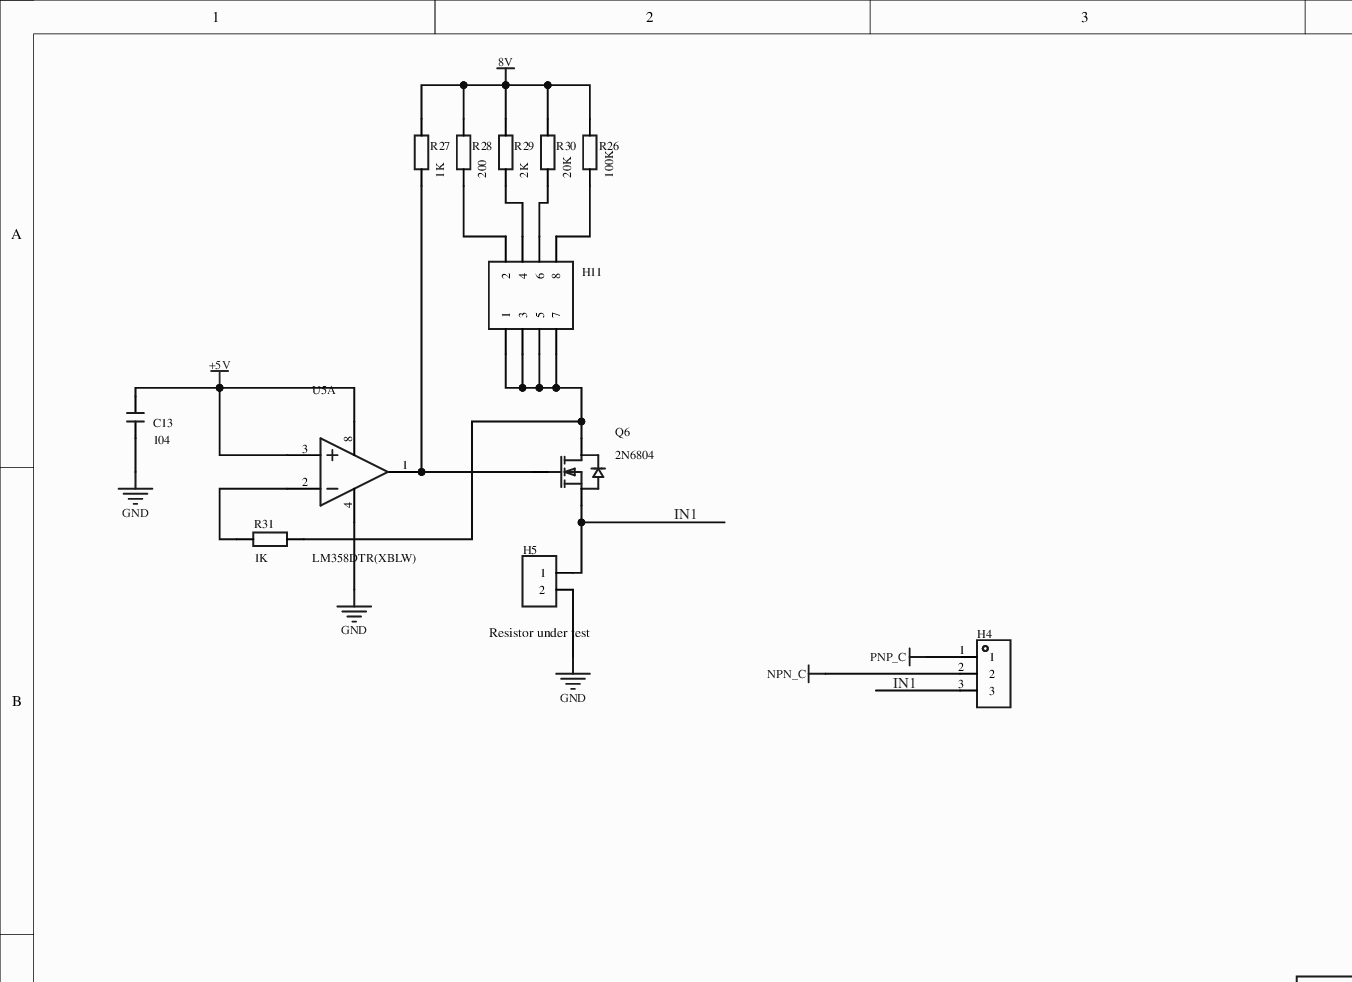
[diagram p0: MISC52056-3.schdoc, top left]
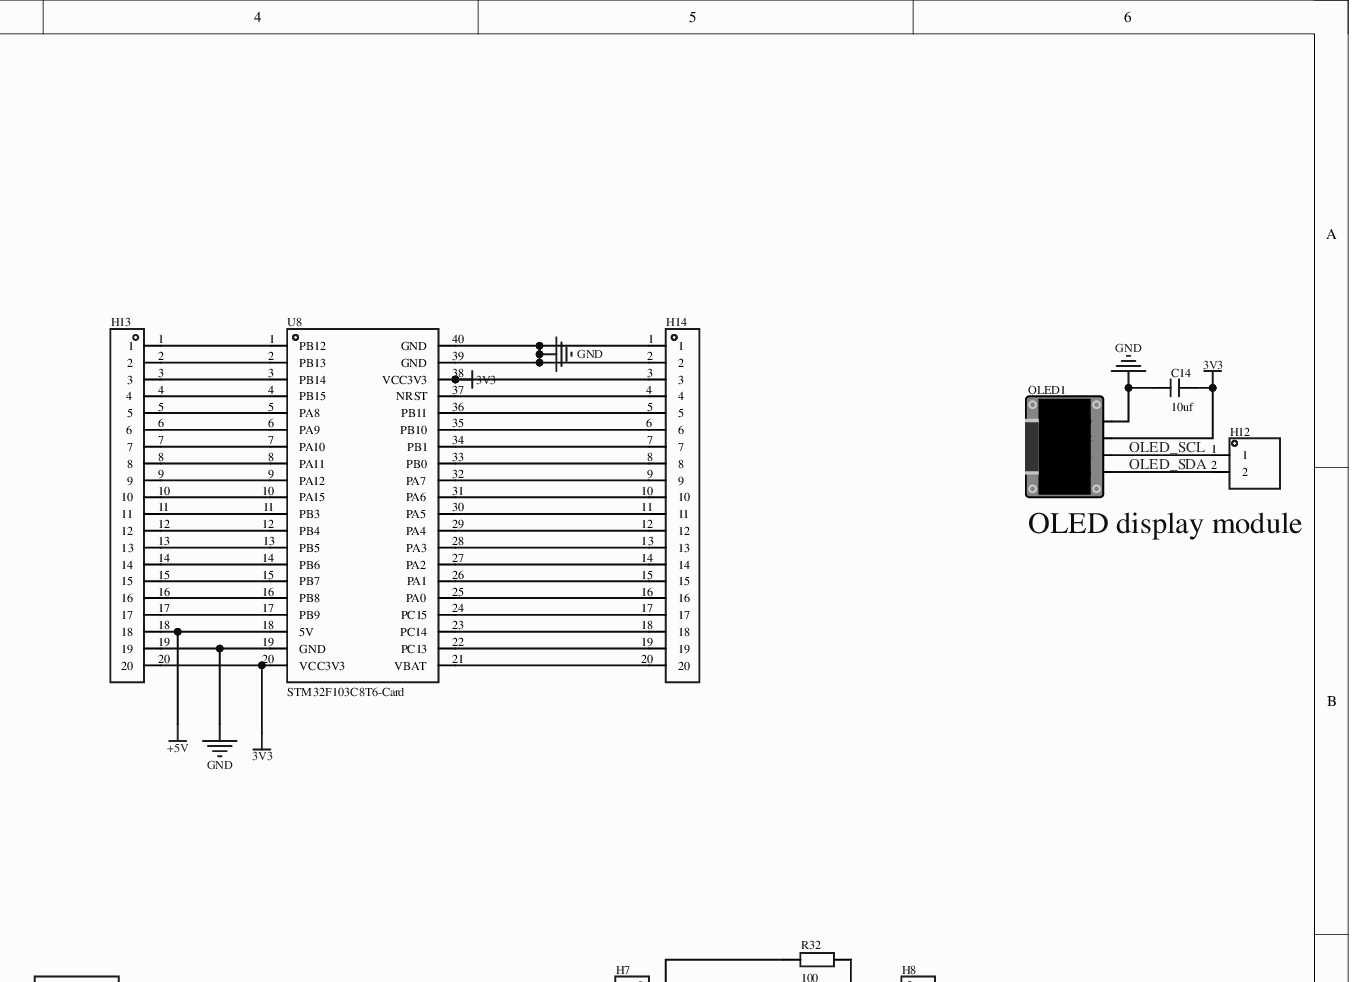
[diagram p1: MISC52056-3.schdoc, top right]
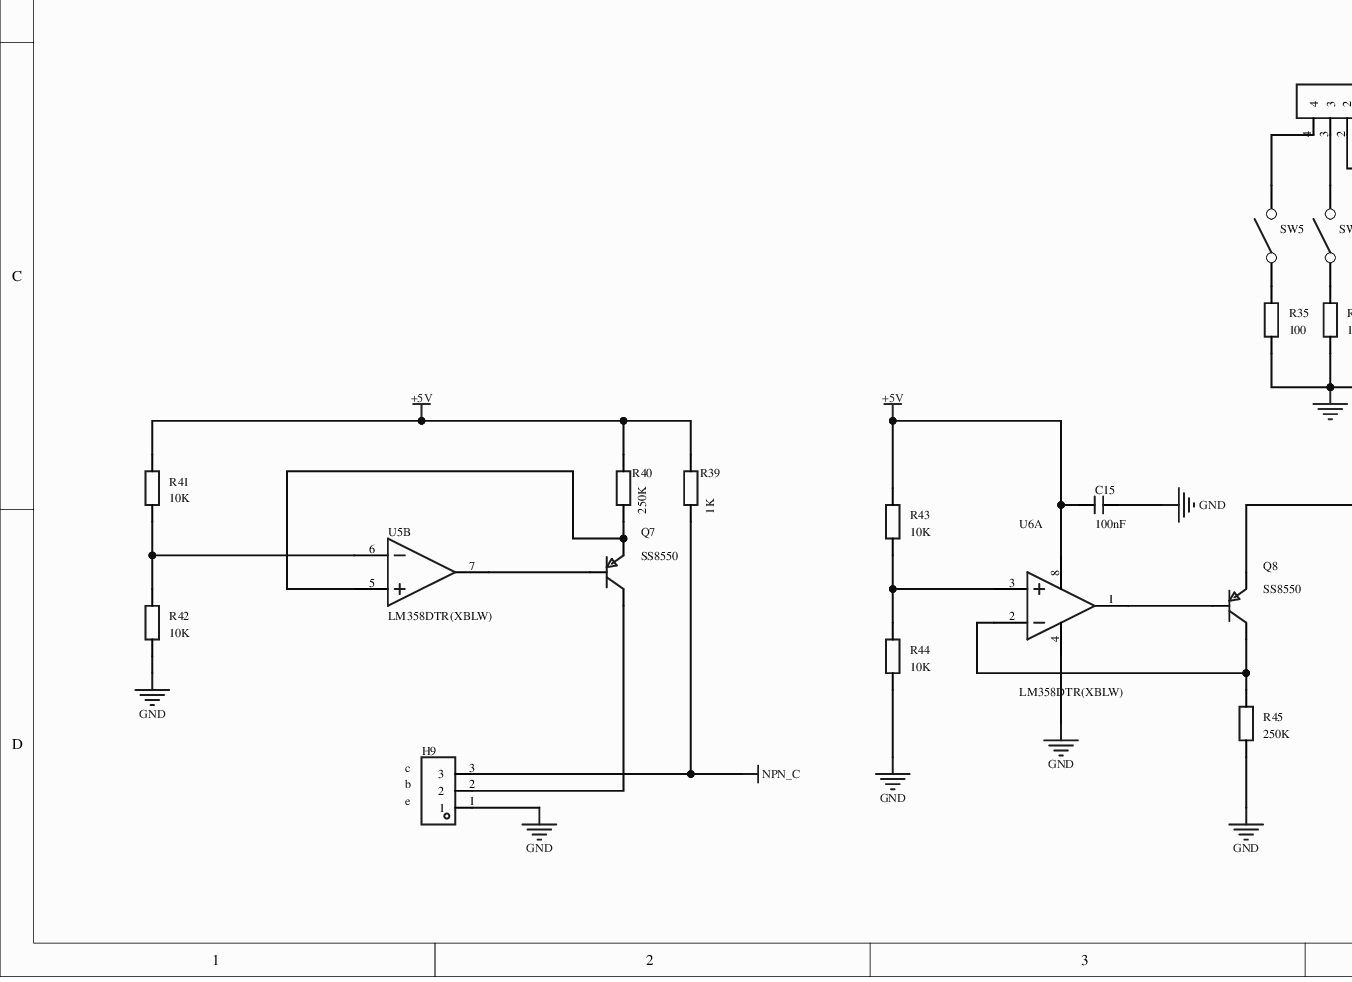
[diagram p2: MISC52056-3.schdoc, bottom left]
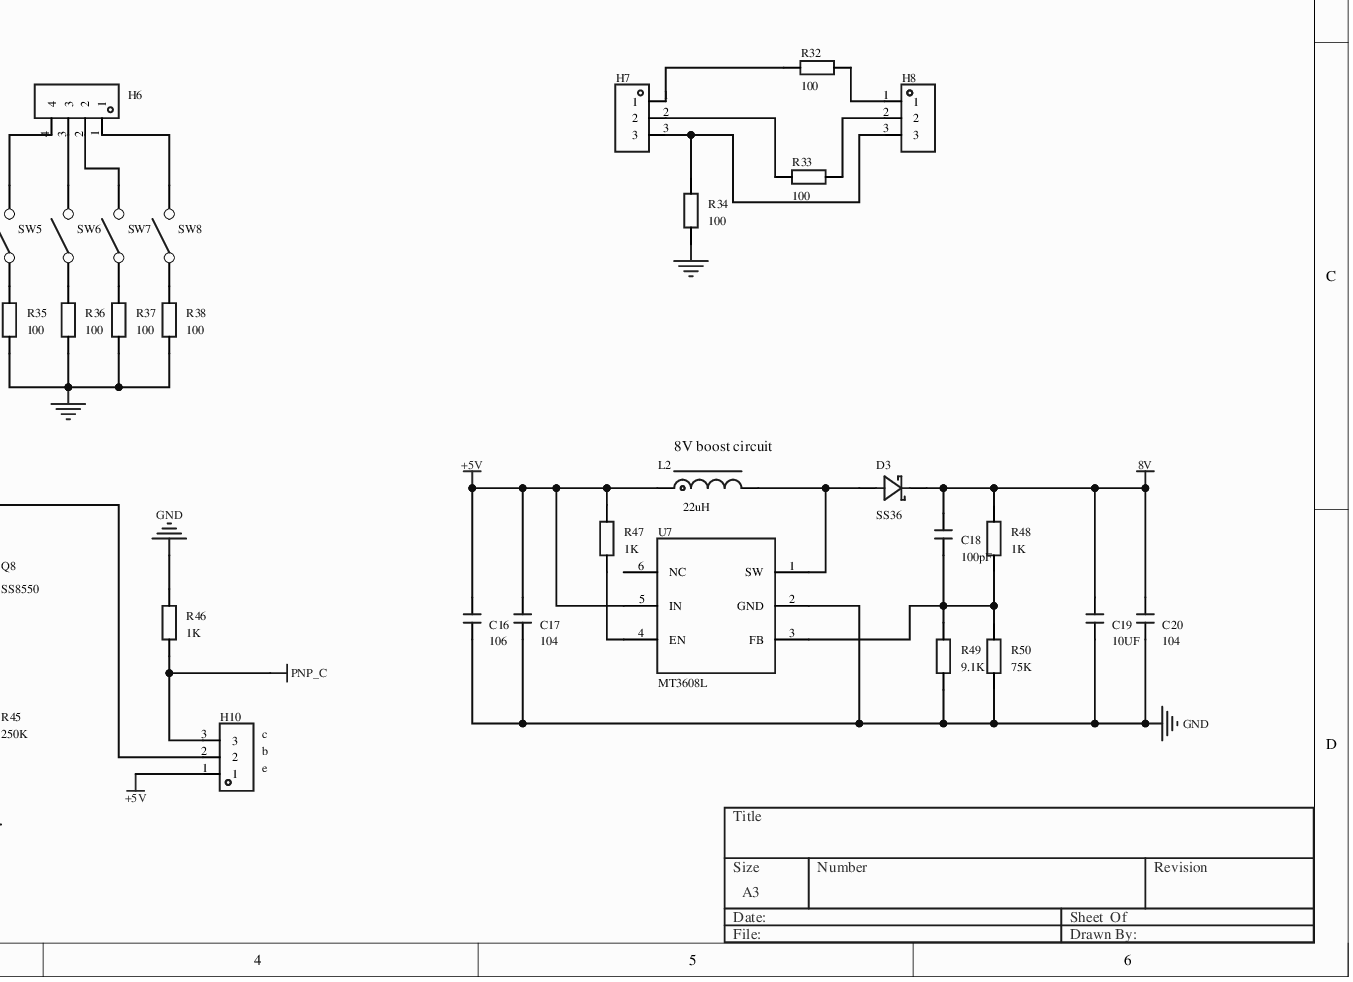
[diagram p3: MISC52056-3.schdoc, bottom right]
# Altium project MISC52056-2.PrjPcb
1 sheet, 58 parts. Net scope: global (net labels, ports and power ports of the same name join across sheets).
Board file: MISC52056.pcbdoc

## Sheet MISC52056-3.schdoc
size 393 x 282 mm; @Page No: 1; @Page Count: 1; @Schematic Name: MISC52056; @Project Name: MISC52056; @Board Name: MISC52056; @Update Date: 2025-02-22; @Create Time: 23:15:00; @Update Time: 00:31:48; @Create Date: 2025-02-22

### Parts
C13  104  [C0603]
C14  10uf  [C0603]
C15  100nF  [C0603]
C16  106  [C0603]
C17  104  [C0603]
C18  100pF  [C0603]
C19  10UF  [C0603]
C20  104  [C0603]
D3  SS36  [SMA_L4.3-W2.6-LS5.0-FD]
H4  (no value)  [HDR-TH_3P-P2.54-V-F]
H5  (no value)  [HDR-TH_2P-P2.54-V-F]
H6  (no value)  [HDR-TH_4P-P2.54-V-M]
H7  (no value)  [HDR-TH_3P-P2.54-V-F]
H8  (no value)  [HDR-TH_3P-P2.54-V-F]
H9  (no value)  [HDR-TH_3P-P2.54-V-F]
H10  (no value)  [HDR-TH_3P-P2.54-V-F]
H11  (no value)  [HDR-TH_8P-P2.54-V-M-R2-C4-S2.54]
H12  (no value)  [HDR-TH_2P-P2.54-V-M-1]
H13  (no value)  [HDR-TH_20P-P2.54-V-M-1]
H14  (no value)  [HDR-TH_20P-P2.54-V-M-1]
L2  22uH  [IND-SMD_L7.1-W6.6]
OLED1  (no value)  [0.96OLED_4P]
Q6  2N6804  [TO-220-3_L10.0-W4.5-P2.54-L]
Q7  SS8550  [SOT-23-3_L2.9-W1.3-P1.90-LS2.4-BR]
Q8  SS8550  [SOT-23-3_L2.9-W1.3-P1.90-LS2.4-BR]
R26  100K  [R0603]
R27  1K  [R0603]
R28  200  [R0603]
R29  2K  [R0603]
R30  20K  [R0603]
R31  1K  [R0603]
R32  100  [R0603]
R33  100  [R0603]
R34  100  [R0603]
R35  100  [R0603]
R36  100  [R0603]
R37  100  [R0603]
R38  100  [R0603]
R39  1K  [R0603]
R40  250K  [R0603]
R41  10K  [R0603]
R42  10K  [R0603]
R43  10K  [R0603]
R44  10K  [R0603]
R45  250K  [R0603]
R46  1K  [R0603]
R47  1K  [R0603]
R48  1K  [R0603]
R49  9.1K  [R0603]
R50  75K  [R0603]
SW5  TS-1088-AR02016  [SW-SMD_L3.9-W3.0-P4.45]  (value not drawn)
SW6  TS-1088-AR02016  [SW-SMD_L3.9-W3.0-P4.45]  (value not drawn)
SW7  TS-1088-AR02016  [SW-SMD_L3.9-W3.0-P4.45]  (value not drawn)
SW8  TS-1088-AR02016  [SW-SMD_L3.9-W3.0-P4.45]  (value not drawn)
U5  LM358DTR(XBLW)  [SOIC-8_L4.9-W4.0-P1.27-LS6.0-BL]  (parts A,B of 2)
U6  LM358DTR(XBLW)  [SOIC-8_L4.9-W4.0-P1.27-LS6.0-BL]  (part A of 2)
U7  MT3608L  [SOT-23-6_L2.9-W1.6-P0.95-LS2.8-BL_3]
U8  STM32F103C8T6-Card  [CONN-TH_L53.3-W22.9_STM32F103C8T6-CARD]

### Nets
3V3: C14.1 H13.20 H14.3 OLED1.2(VCC) U8.20(VCC3V3) U8.38(VCC3V3)
GND: C13.1 C14.2 C15.1 C16.2 C17.2 C19.2 C20.2 H5.2 H9.1 H13.19 H14.1 H14.2 OLED1.1(GND) R34.2 R35.2 R36.2 R37.2 R38.2 R42.1 R44.1 R45.1 R46.2 R49.1 R50.1 U5.4(V-) U6.4(V-) U7.2(GND) U8.19(GND) U8.39(GND) U8.40(GND)  [also labelled 5V, E]
8V: C18.1 C19.1 C20.1 D3.2(K) R26.2 R27.2 R28.2 R29.2 R30.2 R48.1
+5V: C13.2 C15.2 C16.1 C17.1 H10.1 H13.18 L2.1 R39.2 R40.2 R41.2 R43.2 R47.2 U5.3(IN+) U5.8(V+) U6.8(V+) U7.5(IN) U8.18(5V)
NPN_C: H4.1 H4.2 H9.3 H10.3 R39.1 R46.1  [also labelled C, PNP_C]
IN1: H4.3 H5.1 Q6.3(S)
OLED_SCL: H12.1 OLED1.3(SCL)
OLED_SDA: H12.2 OLED1.4(SDA)
NetC18_2: C18.2 R48.2 R49.2 R50.2 U7.3(FB)
NetD3_1: D3.1(A) L2.2 U7.1(SW)
NetH6_1: H6.1 SW8.2(NO)
NetH6_2: H6.2 SW7.2(NO)
NetH6_3: H6.3 SW6.2(NO)
NetH6_4: H6.4 SW5.2(NO)
NetH7_1: H7.1 R32.2
NetH7_2: H7.2 R33.2
NetH7_3: H7.3 H8.3 R34.1
NetH8_1: H8.1 R32.1
NetH8_2: H8.2 R33.1
NetH9_2: H9.2 Q7.3(C)
NetH10_2: H10.2 Q8.2(E)
NetH11_1: H11.1 H11.3 H11.5 H11.7 Q6.2(D) R31.1
NetH11_2: H11.2 R28.1
NetH11_4: H11.4 R29.1
NetH11_6: H11.6 R30.1
NetH11_8: H11.8 R26.1
NetH13_1: H13.1 U8.1(PB12)
NetH13_2: H13.2 U8.2(PB13)
NetH13_3: H13.3 U8.3(PB14)
NetH13_4: H13.4 U8.4(PB15)
NetH13_5: H13.5 U8.5(PA8)
NetH13_6: H13.6 U8.6(PA9)
NetH13_7: H13.7 U8.7(PA10)
NetH13_8: H13.8 U8.8(PA11)
NetH13_9: H13.9 U8.9(PA12)
NetH13_10: H13.10 U8.10(PA15)
NetH13_11: H13.11 U8.11(PB3)
NetH13_12: H13.12 U8.12(PB4)
NetH13_13: H13.13 U8.13(PB5)
NetH13_14: H13.14 U8.14(PB6)
NetH13_15: H13.15 U8.15(PB7)
NetH13_16: H13.16 U8.16(PB8)
NetH13_17: H13.17 U8.17(PB9)
NetH14_4: H14.4 U8.37(NRST)
NetH14_5: H14.5 U8.36(PB11)
NetH14_6: H14.6 U8.35(PB10)
NetH14_7: H14.7 U8.34(PB1)
NetH14_8: H14.8 U8.33(PB0)
NetH14_9: H14.9 U8.32(PA7)
NetH14_10: H14.10 U8.31(PA6)
NetH14_11: H14.11 U8.30(PA5)
NetH14_12: H14.12 U8.29(PA4)
NetH14_13: H14.13 U8.28(PA3)
NetH14_14: H14.14 U8.27(PA2)
NetH14_15: H14.15 U8.26(PA1)
NetH14_16: H14.16 U8.25(PA0)
NetH14_17: H14.17 U8.24(PC15)
NetH14_18: H14.18 U8.23(PC14)
NetH14_19: H14.19 U8.22(PC13)
NetH14_20: H14.20 U8.21(VBAT)
NetQ6_1: Q6.1(G) R27.1 U5.1(OUT)
NetQ7_1: Q7.1(B) U5.7(OUT_B)
NetQ7_2: Q7.2(E) R40.1 U5.5(IN_B+)
NetQ8_1: Q8.1(B) U6.1(OUT)
NetQ8_3: Q8.3(C) R45.2 U6.2(IN-)
NetR31_2: R31.2 U5.2(IN-)
NetR35_1: R35.1 SW5.1(COMMON)
NetR36_1: R36.1 SW6.1(COMMON)
NetR37_1: R37.1 SW7.1(COMMON)
NetR38_1: R38.1 SW8.1(COMMON)
NetR41_1: R41.1 R42.2 U5.6(IN_B-)
NetR43_1: R43.1 R44.2 U6.3(IN+)
NetR47_1: R47.1 U7.4(EN)

Not connected (* = marked no-connect by the designer): U7 6(NC)

### Notes on the sheet
- OLED display module
- (near H5) Resistor under test
- (near L2) 8V boost circuit
- (near H10) c
- (near H10) b
- (near H9) c
- (near H9) b
- (near H9) e
- (near H10) e
- Title
- File:
- Date:
- Size
- A3
- Number
- Drawn By:
- Sheet
- Of
- Revision

### Library data of the parts
C13-C20 = CAP_0603: ConvertToPcb: yes; SymbolName: CapAcitance; ModelId: ac125912035d415993ca9572d50418b1; ModelName: C0603_L1.6-W0.8-H0.8; ModelTransform: 62.992,31.496,0,0,0,0,0,0,0; Device: CAP_0603; AddInBom: yes; Supplier Footprint: 0603; FootprintName: C0603
  C13 C17 C20: Value: 104
  C14: Value: 10uf
  C15: Value: 100nF
  C16: Value: 106
  C18: Value: 100pF
  C19: Value: 10UF
D3 = SS36_C7420367: Diode configuration: discrete; forward voltage drop (Vf): 700mV@3.0A; DC reverse voltage (Vr): 60V; rectifier current: 3A;; Manufacturer: 宏迦橙; AddInBom: yes; ModelId: 7e24bebe6cd74171ae8c9de6fc5b78aa; ModelTransform: 198.4248,103.5431,0,180,0,0,0,0,0; Reverse Leakage Current (Ir): 10mA@60V; Symbol: SS36_C7420367; Device: SS36_C7420367; LCSC Part Name: 电压:60V 电流:3A; SupplierPart: C7420367; ManufacturerPart: SS36; Supplier Footprint: SMA(DO-214AC); JLCPCB Part Class: Extended library; Datasheet: example.com/20230828/75438452AEE6C276EDA92B2AF599BE05.pdf; Supplier: LCSC; ConvertToPcb: yes; FootprintName: SMA_L4.3-W2.6-LS5.0-FD; ModelName: SMA_L4.3-W2.6-LS5.0-FD; Diode Configuration: Discrete; Forward Voltage (Vf@If): 700mV@3.0A; Reverse Voltage (Vr): 60V; Rectified Current: 3A
H4 H7-H10 = HDR-F_2.54_1x3P: Symbol: PM254V-11-03-H85; ConvertToPcb: yes; ModelId: f3b3cc5aae9641bf9e56fc160cef875b; ModelName: HDR2.54-F-LI-1X3P; ModelTransform: 299.9994,100,0,0,0,0,0,0,-118.11; Device: HDR-F_2.54_1x3P; AddInBom: yes; SupplierPart: C541850; Supplier Footprint: 插件; FootprintName: HDR-TH_3P-P2.54-V-F
H5 = HDR-F_2.54_1x2P: Symbol: Header-Female-2.54_1x2; ConvertToPcb: yes; ModelId: a9450ef445564560a104363b9aacde4e; ModelName: HDR-TH_2P-P2.54-F-LI-1X2P; ModelTransform: 215.7476,98.425,0,0,0,0,0,0,-129.921; Device: HDR-F_2.54_1x2P; AddInBom: yes; SupplierPart: C49661; Supplier Footprint: 插件; FootprintName: HDR-TH_2P-P2.54-V-F
H6 = HDR-M_2.54_1x4P: Symbol: PZ254V-11-04P; ConvertToPcb: yes; ModelId: 112f4d05e8d64e99ab9a333894bea4f9; ModelName: HDR-TH_4P-P2.54-M-LI-1X4P; ModelTransform: 399.999,104.7242,0,0,0,0,0,0,-118.11; Device: HDR-M_2.54_1x4P; AddInBom: yes; SupplierPart: C492403; Supplier Footprint: 插件; FootprintName: HDR-TH_4P-P2.54-V-M
H11 = HDR-M_2.54_2x4: Symbol: HDR-M-2.54_2x4; ConvertToPcb: yes; ModelId: 9655140a9899454ea9d6a6732d55fb0e; ModelName: HDR-TH_8P-P2.54-M-LI-2X4P; ModelTransform: 399.999,200,0,0,0,0,0,0,-118.11; Device: HDR-M_2.54_2x4; AddInBom: yes; SupplierPart: C124386; Supplier Footprint: 插件,P=2.54mm; FootprintName: HDR-TH_8P-P2.54-V-M-R2-C4-S2.54
H12 = HDR-M_2.54_1x2P: Symbol: 210S-1*2P L=11.6MMGold-plated black; ConvertToPcb: yes; ModelId: 79b2e9f2d70a4d68a1b7098f27c6d4c5; ModelName: HDR-M-2.54_1x2; ModelTransform: 200,100,0,0,0,0,0,0,-118.11; Device: HDR-M_2.54_1x2P; AddInBom: yes; SupplierPart: C124375; Supplier Footprint: 插件; FootprintName: HDR-TH_2P-P2.54-V-M-1
H13 H14 = HDR-M_2.54_1x20P: Pitch: 2.54mm; total pin count: 20; rows: 1; pin structure: -; row spacing: -; mounting type: through-hole; round/square pin: -; rated current: -; rated voltage: -; mating pin length: -; plastic height: -; contact material: brass; contact plating: -; colour: black;; Symbol: HDR_2.54-1x20P; ConvertToPcb: yes; ModelId: f68709be121d406db68b06f32a595389; ModelName: HDR-M-2.54_1x20; ModelTransform: 1999.996,100,0,0,0,0,0,0,-118.11; Device: HDR-M_2.54_1x20P; AddInBom: yes; SupplierPart: C50981; Supplier Footprint: 插件; FootprintName: HDR-TH_20P-P2.54-V-M-1
L2 = YSPI0630A-220M: Inductance: 22uH; tolerance: ±20%; rated current: 3A;; Manufacturer: YJYCOIN(益嘉源); AddInBom: yes; DC Resistance (DCR): 130mΩ; ModelId: f4ba7fb6b518404398a5bef98cb0da31; ModelName: IND-SMD_L6.6-W7.1-H3.0; ModelTransform: 275.59,263.779,0,0,0,0,0,0.0005,0; Symbol: YSPI0630A-220M; Device: YSPI0630A-220M; LCSC Part Name: 22uH ±20%; SupplierPart: C497873; ManufacturerPart: YSPI0630A-220M; Supplier Footprint: SMD,6.6x7.1mm; Datasheet: example.com/20200317/C497869_D09F597887D5FB8B541C5C98B400E286.pdf; Supplier: LCSC; ConvertToPcb: yes; Value: 22uH; Tolerance: ±20%; Rated Current: 3A; FootprintName: IND-SMD_L7.1-W6.6
OLED1 = 0.96OLED模块_4P: Device: 0.96OLED module_4P; ConvertToPcb: yes; ModelId: 79c000fdb68d45a296c2e9bedf4f9055; ModelTransform: 1393.69792,1318.895,0,0,0,0,0,-560.079,-137.795; AddInBom: yes; SymbolName: 0.96OLED module_4P; FootprintName: 0.96OLED_4P; Supplier Footprint: 插件; ModelName: 0.96OLED_4P
Q6 = IRFZ44NPBF: Type: 1 N-channel; drain-source voltage (Vdss): 55V; continuous drain current (Id): 49A; on-resistance (RDS(on)@Vgs,Id): 17.5mΩ@10V,25A; power (Pd): 94W; threshold voltage (Vgs(th)@Id): 4V@250uA;; Manufacturer: Infineon(英飞凌); AddInBom: yes; ModelId: b3c9e38e4428458f8b925050989b538f; ModelTransform: 397.637,177.165,0,180,0,0,-0.004,19.88,-78.74; Total Gate Charge (Qg@Vgs): 63nC; Input Capacitance (Ciss@Vds): 1.47nF; Reverse Transfer Capacitance (Crss@Vds): 88pF; Symbol: IRFZ44NPBF; Manufacturer Part: 2N6804; Device: IRFZ44NPBF; LCSC Part Name: 1个N沟道 耐压:55V 电流:49A; SupplierPart: C2586; Supplier Footprint: TO-220-3; JLCPCB Part Class: Extended library; Datasheet: example.com/20120403/1457706463862.pdf; Supplier: LCSC; ConvertToPcb: yes; FootprintName: TO-220-3_L10.0-W4.5-P2.54-L; ModelName: TO-220-3_L10.0-W4.5-P2.54-L; Drain Source Voltage (Vdss): 55V; Continuous Drain Current (Id): 49A; Drain Source On Resistance (RDS(on)@Vgs,Id): 17.5mΩ@10V,25A; Power Dissipation (Pd): 94W; Gate Threshold Voltage (Vgs(th)@Id): 4V@250uA; Operating Temperature: -55℃~+175℃
Q7 Q8 = SS8550_C7420371: Transistor type: PNP; collector current (Ic): 1.5A; collector-emitter breakdown voltage (Vceo): 25V; power (Pd): 300mW; DC current gain (hFE@Ic,Vce): 120@100mA,1.0V;; Manufacturer: 宏迦橙; AddInBom: yes; Transition Frequency (fT): 100MHz; Collector Cut-Off Current (Icbo): 100nA; Collector-Emitter Saturation Voltage (VCE(sat)@Ic,Ib): 500mV@800mA,80mA; ModelId: c62791f0466c4ae2a892c056b845b0ca; ModelName: SOT-23-3P_L2.9-W1.3-H1.0-LS2.4-P0.95; ModelTransform: 98.425,114.173,0,180,0,0,0.0005,-0.0005,0; Symbol: SS8550_C7420371; Device: SS8550_C7420371; LCSC Part Name: 耐压:25V 电流:1.5A PNP H档 200-350; SupplierPart: C7420371; ManufacturerPart: SS8550; Supplier Footprint: SOT-23; JLCPCB Part Class: Extended library; Datasheet: example.com/20231222/5BDA6DBF3A79C59009F81F0EEE6F8969.pdf; Supplier: LCSC; ConvertToPcb: yes; Transistor Type: PNP; Collector Current (Ic): 1.5A; Collector-Emitter Breakdown Voltage (Vceo): 25V; Power Dissipation (Pd): 300mW; DC Current Gain (hFE@Ic,Vce): 120@100mA,1.0V; Operating Temperature: -55℃~+150℃; FootprintName: SOT-23-3_L2.9-W1.3-P1.90-LS2.4-BR
R26-R50 = Res_0603: ConvertToPcb: yes; SymbolName: Resistor; ModelId: fc143cca1e79419f9cd78b61e9279f08; ModelTransform: 31.8897,63.7794,0,90,0,0,0,0,0; Device: Res_0603; AddInBom: yes; Supplier Footprint: 0603; FootprintName: R0603; ModelName: R0603
  R26: Value: 100K
  R27 R31 R39 R46-R48: Value: 1K
  R28: Value: 200
  R29: Value: 2K
  R30: Value: 20K
  R32-R38: Value: 100
  R40 R45: Value: 250K
  R41-R44: Value: 10K
  R49: Value: 9.1K
  R50: Value: 75K
SW5-SW8 = TS-1088-AR02016: 电路结构:单刀单掷;按钮形状:圆形按钮;作用力:160gf;安装方式:立贴;开关长度:4mm;开关宽度:3mm;开关高度:2mm;带支架:不带;触点电流:50mA;额定电压(DC):12V;绝缘电阻:100MΩ;机械寿命:10万次;; Manufacturer: XUNPU(讯普); AddInBom: yes; Circuit: SPST; Actuator Style: Round button; Operating Force: 160gf; Switch Length: 4mm; Switch Width: 3mm; Switch Height: 2mm; Strike Gundam: None; Contact Current: 50mA; Voltage Rating (DC): 12V; Insulation Resistance: 100MΩ; Actuator/Cap Color: Black; Pin Style: SMD tab; Mechanical Life: 10万 cycles; ModelId: b26698b69f274ffabef8a26c7d0e5dd1; ModelName: SW-SMD_L3.9-W2.9-H2.0-LS4.8; ModelTransform: 188.976,114.174,0,0,0,0,0,0,0; Symbol: TS-1088-AR02016; Device: TS-1088-AR02016; LCSC Part Name: 4*3*2mm 立贴 轻触开关; SupplierPart: C720477; ManufacturerPart: TS-1088-AR02016; Supplier Footprint: SMD; JLCPCB Part Class: Extended library; Datasheet: example.com/20200810/C720475_60D09DD6C54279ADDB2DC25100F1CC11.pdf; Supplier: LCSC; ConvertToPcb: yes; Mounting Style: Upright SMD; Operating Temperature: -30℃~+80℃; FootprintName: SW-SMD_L3.9-W3.0-P4.45
U5 U6 = LM358DTR(XBLW): Amplifier count: dual; gain-bandwidth product (GBP): 1MHz; input bias current (Ib): 45nA; input offset voltage (Vos): 7mV;; Manufacturer: XBLW(芯伯乐); Relevance: []; AddInBom: yes; Supply Voltage: 3V~24V; ModelId: f04b1702bced497a80c713fe4e712e0c; ModelTransform: 192.913,238.9759,0,0,0,0,0,0,0; Symbol: LM358DTR(XBLW); Device: LM358DTR(XBLW); LCSC Part Name: LM358DTR; SupplierPart: C18723608; ManufacturerPart: LM358DTR(XBLW); Supplier Footprint: SOP-8; JLCPCB Part Class: Extended library; Datasheet: example.com/20231019/5D5266BD565DC949181482F46BBEC63B.pdf; Supplier: LCSC; ConvertToPcb: yes; Number of Circuits: Dual; Gain Bandwidth Product(GBP): 1MHz; Current - Input Bias(Ib): 45nA; Voltage - Input Offset(Vos): 7mV; FootprintName: SOIC-8_L4.9-W4.0-P1.27-LS6.0-BL; ModelName: SOIC-8_L4.9-W4.0-P1.27-LS6.0-BL
U7 = MT3608L: Operating voltage: 2.2V~16V; output current: 2.5A;; Manufacturer: 西安航天民芯; AddInBom: yes; Number of Outputs: 1; ModelId: fb8f66c7218e47258c3712467298ba04; ModelTransform: 114.173,110.236,0,0,0,0,0,0,0; Symbol: MT3608L; Device: MT3608L; LCSC Part Name: 高效2.5A 1.2MHz升压转换器; SupplierPart: C2932326; ManufacturerPart: MT3608L; Supplier Footprint: SOT-23-6; JLCPCB Part Class: Extended library; Datasheet: example.com/20211213/953A62CC1033762E00AABAD4906DD7F1.pdf; Supplier: LCSC; ConvertToPcb: yes; Input Voltage: 2.2V~16V; Output Current: 2.5A; FootprintName: SOT-23-6_L2.9-W1.6-P0.95-LS2.8-BL_3; ModelName: SOT-23-6_L2.9-W1.6-P0.95-LS2.8-BL_3
U8 = STM32F103C8T6-Card: AddInBom: yes; Symbol: STM32F103C8T6-CARD; Device: STM32F103C8T6-Card; LCSC Part Name: STM32F103C8T6-Card; SupplierPart: C9900077949; ManufacturerPart: STM32F103C8T6-Card; Supplier Footprint: 插件; Supplier: LCSC; ConvertToPcb: yes; FootprintName: CONN-TH_L53.3-W22.9_STM32F103C8T6-CARD